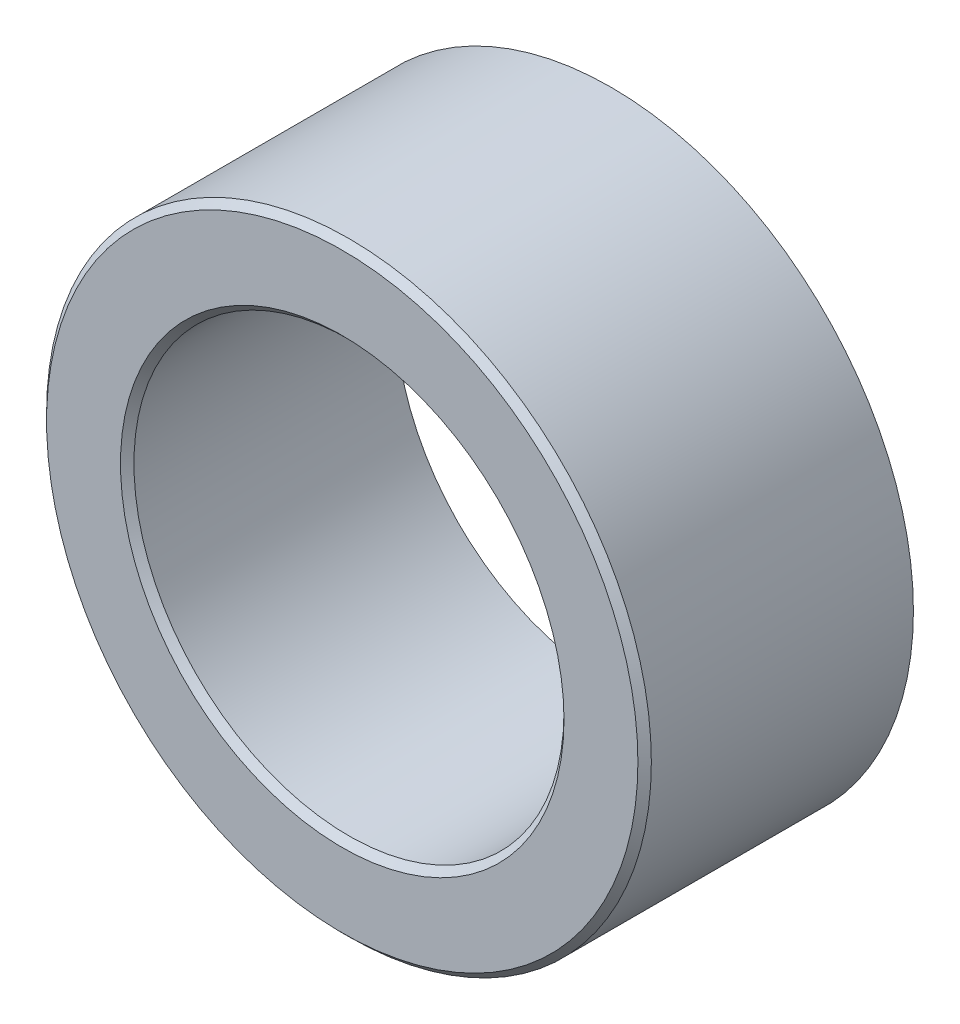
from build123d import *

# Parameters (mm, degrees)
SKETCH_1_R          = 22.5
EXTRUDE_1_DEPTH     = 20
SKETCH_2_R          = 16
CUT_EXTRUDE_1_DEPTH = 20
CHAMFER_1_SIZE      = 0.5
CHAMFER_2_SIZE      = 0.5


with BuildPart() as part:
    # 草图1 → 凸台-拉伸1 (new body)
    with BuildSketch(Plane.XY):
        Circle(SKETCH_1_R)
    extrude(amount=EXTRUDE_1_DEPTH)

    # 草图2 → 切除-拉伸1 (cut)
    with BuildSketch(Plane.XY.offset(20)):
        Circle(SKETCH_2_R)
    extrude(amount=-CUT_EXTRUDE_1_DEPTH, mode=Mode.SUBTRACT)

    # 倒角1
    chamfer_1_edges = [part.edges().sort_by_distance(p)[0] for p in [
        (-16, 0, 20),
    ]]
    chamfer(chamfer_1_edges, length=CHAMFER_1_SIZE)

    # 倒角2
    chamfer_2_edges = [part.edges().sort_by_distance(p)[0] for p in [
        (-22.5, 0, 20),
    ]]
    chamfer(chamfer_2_edges, length=CHAMFER_2_SIZE)


solid = part.part
